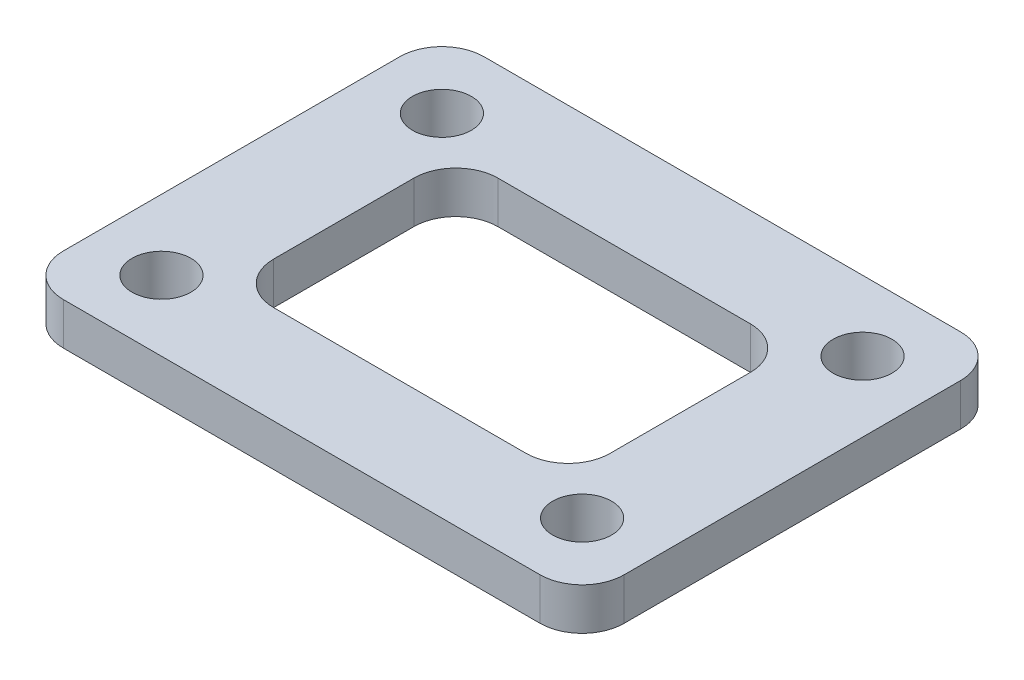
from build123d import *

# Parameters (mm, degrees)
SKETCH_1_R      = 2.1
EXTRUDE_1_DEPTH = 3


with BuildPart() as part:
    # 草图1 → 凸台-拉伸1 (new body)
    with BuildSketch(Plane(origin=(0, 0, 0), x_dir=(1, 0, 0), z_dir=(0, 1, 0))):
        with BuildLine():
            Line((-17, -15), (17, -15))
            ThreePointArc((17, -15), (19.121320344, -14.121320344), (20, -12))
            Line((20, -12), (20, 12))
            ThreePointArc((20, 12), (19.121320344, 14.121320344), (17, 15))
            Line((17, 15), (-17, 15))
            ThreePointArc((-17, 15), (-19.121320344, 14.121320344), (-20, 12))
            Line((-20, 12), (-20, -12))
            ThreePointArc((-20, -12), (-19.121320344, -14.121320344), (-17, -15))
        make_face()
        with Locations(Location((-15, 10, 0), (0, 0, 270))):
            Circle(SKETCH_1_R, mode=Mode.SUBTRACT)
        with Locations(Location((15, 10, 0), (0, 0, 270))):
            Circle(SKETCH_1_R, mode=Mode.SUBTRACT)
        with Locations(Location((-15, -10, 0), (0, 0, 270))):
            Circle(SKETCH_1_R, mode=Mode.SUBTRACT)
        with Locations(Location((15, -10, 0), (0, 0, 270))):
            Circle(SKETCH_1_R, mode=Mode.SUBTRACT)
        with BuildLine():
            Line((-9, -8), (9, -8))
            ThreePointArc((9, -8), (11.121320344, -7.121320344), (12, -5))
            Line((12, -5), (12, 5))
            ThreePointArc((12, 5), (11.121320344, 7.121320344), (9, 8))
            Line((9, 8), (-9, 8))
            ThreePointArc((-9, 8), (-11.121320344, 7.121320344), (-12, 5))
            Line((-12, 5), (-12, -5))
            ThreePointArc((-12, -5), (-11.121320344, -7.121320344), (-9, -8))
        make_face(mode=Mode.SUBTRACT)
    extrude(amount=EXTRUDE_1_DEPTH)


solid = part.part
